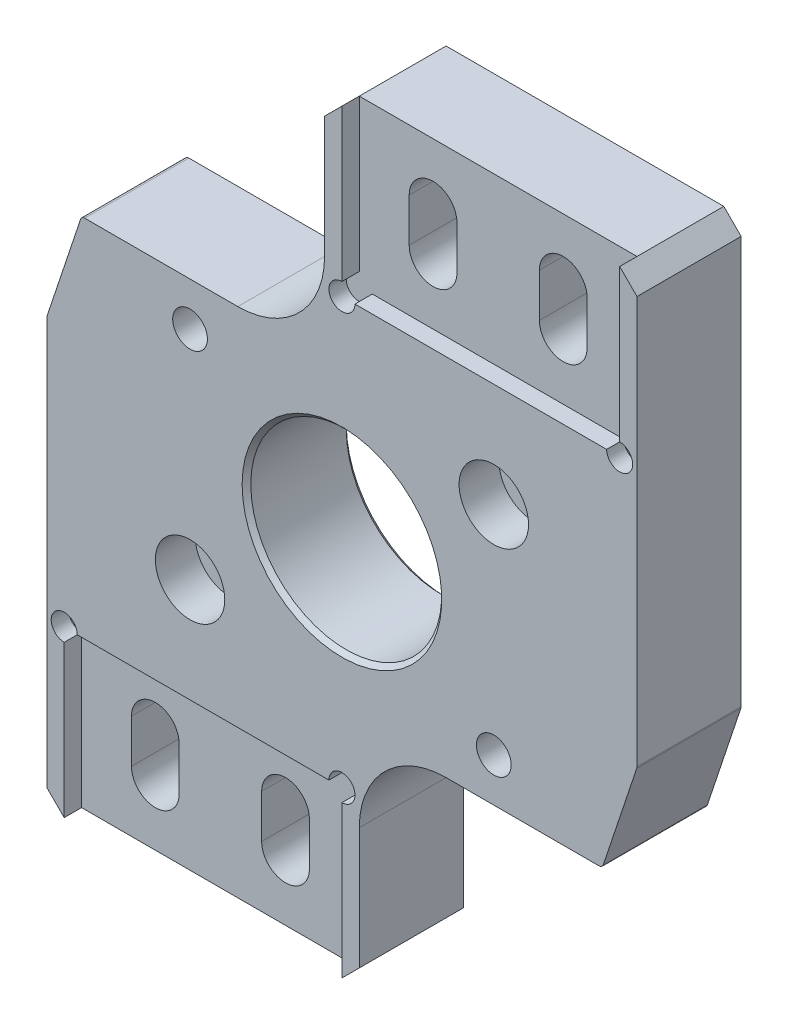
from build123d import *
from OCP.BRepFilletAPI import BRepFilletAPI_MakeChamfer

# Parameters (mm, degrees)
SKETCH1_W                                            = 68
SKETCH1_H                                            = 87
BOSS_EXTRUDE1_DEPTH                                  = 12
SKETCH3_R                                            = 11
SKETCH3_W                                            = 32
SKETCH3_H                                            = 26
CUT_EXTRUDE2_DEPTH                                   = 57.5
CUT_EXTRUDE5_DEPTH                                   = 2
FILLET1_R                                            = 10
CHAMFER1_SIZE                                        = 2
CUT_EXTRUDE6_DEPTH                                   = 57.5
CHAMFER2_SIZE                                        = 12
CHAMFER2_SIZE2                                       = 4
FILLET3_R                                            = 0.5
HOLE_SIZE_BY_SOCKET_HEAD_CAP_SCREW_TYPE1_D           = 4.5
HOLE_SIZE_BY_SOCKET_HEAD_CAP_SCREW_TYPE1_CBORE_D     = 8
HOLE_SIZE_BY_SOCKET_HEAD_CAP_SCREW_TYPE1_CBORE_DEPTH = 4.6
SKETCH15_R                                           = 2
CUT_EXTRUDE4_DEPTH                                   = 25
CHAMFER3_SIZE                                        = 0.5


with BuildPart() as part:
    # Sketch1 → Boss-Extrude1 (new body)
    with BuildSketch(Plane.XY):
        Rectangle(SKETCH1_W, SKETCH1_H)
    extrude(amount=BOSS_EXTRUDE1_DEPTH)

    # Sketch3 → Cut-Extrude2 (cut, through all)
    with BuildSketch(Plane.XY.offset(12)):
        Circle(SKETCH3_R)
        with Locations((-18, 30.5)):
            Rectangle(SKETCH3_W, SKETCH3_H)
        with Locations((18, -30.5)):
            Rectangle(SKETCH3_W, SKETCH3_H)
    extrude(amount=-CUT_EXTRUDE2_DEPTH, mode=Mode.SUBTRACT)

    # Sketch16 → Cut-Extrude5 (cut)
    with BuildSketch(Plane.XY.offset(12)):
        with BuildLine():
            Line((0, -43.5), (-32, -43.5))
            Line((-32, -43.5), (-32, -26))
            ThreePointArc((-32, -26), (-33.060660172, -23.439339828), (-30.5, -24.5))
            Line((-30.5, -24.5), (-1.5, -24.5))
            ThreePointArc((-1.5, -24.5), (1.060660172, -23.439339828), (0, -26))
            Line((0, -26), (0, -43.5))
        make_face()
        with BuildLine():
            Line((32, 43.5), (0, 43.5))
            Line((0, 43.5), (0, 26))
            ThreePointArc((0, 26), (-1.060660172, 23.439339828), (1.5, 24.5))
            Line((1.5, 24.5), (30.5, 24.5))
            ThreePointArc((30.5, 24.5), (33.060660172, 23.439339828), (32, 26))
            Line((32, 26), (32, 43.5))
        make_face()
    extrude(amount=-CUT_EXTRUDE5_DEPTH, mode=Mode.SUBTRACT)

    # Fillet1
    fillet1_edges = [part.edges().sort_by_distance(p)[0] for p in [
        (-2, 17.5, 6),
        (2, -17.5, 6),
    ]]
    fillet(fillet1_edges, radius=FILLET1_R)

    # Chamfer1
    chamfer1_edges = [part.edges().sort_by_distance(p)[0] for p in [
        (-34, -43.5, 6),
        (2, -43.5, 6),
        (34, 43.5, 6),
        (-2, 43.5, 6),
    ]]
    chamfer(chamfer1_edges, length=CHAMFER1_SIZE)

    # Sketch17 → Cut-Extrude6 (cut, through all)
    with BuildSketch(Plane(origin=(0, 0, 0), x_dir=(-1, 0, 0), z_dir=(0, 0, -1))):
        with BuildLine():
            Line((-20.75, 36.5), (-20.75, 31.5))
            ThreePointArc((-20.75, 31.5), (-23.5, 28.75), (-26.25, 31.5))
            Line((-26.25, 31.5), (-26.25, 36.5))
            ThreePointArc((-26.25, 36.5), (-23.5, 39.25), (-20.75, 36.5))
        make_face()
        with BuildLine():
            Line((-5.75, 36.5), (-5.75, 31.5))
            ThreePointArc((-5.75, 31.5), (-8.5, 28.75), (-11.25, 31.5))
            Line((-11.25, 31.5), (-11.25, 36.5))
            ThreePointArc((-11.25, 36.5), (-8.5, 39.25), (-5.75, 36.5))
        make_face()
        with BuildLine():
            Line((26.25, -31.5), (26.25, -36.5))
            ThreePointArc((26.25, -36.5), (23.5, -39.25), (20.75, -36.5))
            Line((20.75, -36.5), (20.75, -31.5))
            ThreePointArc((20.75, -31.5), (23.5, -28.75), (26.25, -31.5))
        make_face()
        with BuildLine():
            Line((11.25, -31.5), (11.25, -36.5))
            ThreePointArc((11.25, -36.5), (8.5, -39.25), (5.75, -36.5))
            Line((5.75, -36.5), (5.75, -31.5))
            ThreePointArc((5.75, -31.5), (8.5, -28.75), (11.25, -31.5))
        make_face()
    extrude(amount=-CUT_EXTRUDE6_DEPTH, mode=Mode.SUBTRACT)

    # Chamfer2: one chamfer whose edges measure the first distance from different faces: ONE call of the kernel's chamfer builder (chamfer() names one face for all edges)
    chamfer2_edges_1 = [part.edges().sort_by_distance(p)[0] for p in [
        (-34, 17.5, 6),
    ]]
    chamfer2_side_1 = [part.faces().sort_by_distance(p)[0] for p in [
        (-34, -12, 6),
    ]]
    chamfer2_edges_2 = [part.edges().sort_by_distance(p)[0] for p in [
        (34, -17.5, 6),
    ]]
    chamfer2_side_2 = [part.faces().sort_by_distance(p)[0] for p in [
        (34, 12, 6),
    ]]
    chamfer2 = BRepFilletAPI_MakeChamfer(part.part.solid().wrapped)
    for e in chamfer2_edges_1:
        chamfer2.Add(CHAMFER2_SIZE, CHAMFER2_SIZE2, e.wrapped, chamfer2_side_1[0].wrapped)  # the first distance lies on this face
    for e in chamfer2_edges_2:
        chamfer2.Add(CHAMFER2_SIZE, CHAMFER2_SIZE2, e.wrapped, chamfer2_side_2[0].wrapped)  # the first distance lies on this face
    add(Compound.cast(chamfer2.Shape()), mode=Mode.REPLACE)

    # Fillet3
    fillet3_edges = [part.edges().sort_by_distance(p)[0] for p in [
        (30, -17.5, 6),
        (34, -5.5, 6),
        (-30, 17.5, 6),
        (-34, 5.5, 6),
    ]]
    fillet(fillet3_edges, radius=FILLET3_R)

    # Hole size by socket head cap screw type1 (through all)
    with Locations(Plane.XY.offset(12)):
        with Locations((17.5, 12.5), (-17.5, -12.5)):
            CounterBoreHole(HOLE_SIZE_BY_SOCKET_HEAD_CAP_SCREW_TYPE1_D / 2, HOLE_SIZE_BY_SOCKET_HEAD_CAP_SCREW_TYPE1_CBORE_D / 2, HOLE_SIZE_BY_SOCKET_HEAD_CAP_SCREW_TYPE1_CBORE_DEPTH)

    # Sketch15 → Cut-Extrude4 (cut)
    with BuildSketch(Plane.XY.offset(12)):
        with Locations((17.5, -12.5)):
            Circle(SKETCH15_R)
        with Locations((-17.5, 12.5)):
            Circle(SKETCH15_R)
    extrude(amount=-CUT_EXTRUDE4_DEPTH, mode=Mode.SUBTRACT)

    # Chamfer3
    chamfer3_edges = [part.edges().sort_by_distance(p)[0] for p in [
        (-11, 0, 0),
        (-11, 0, 12),
    ]]
    chamfer(chamfer3_edges, length=CHAMFER3_SIZE)


solid = part.part
